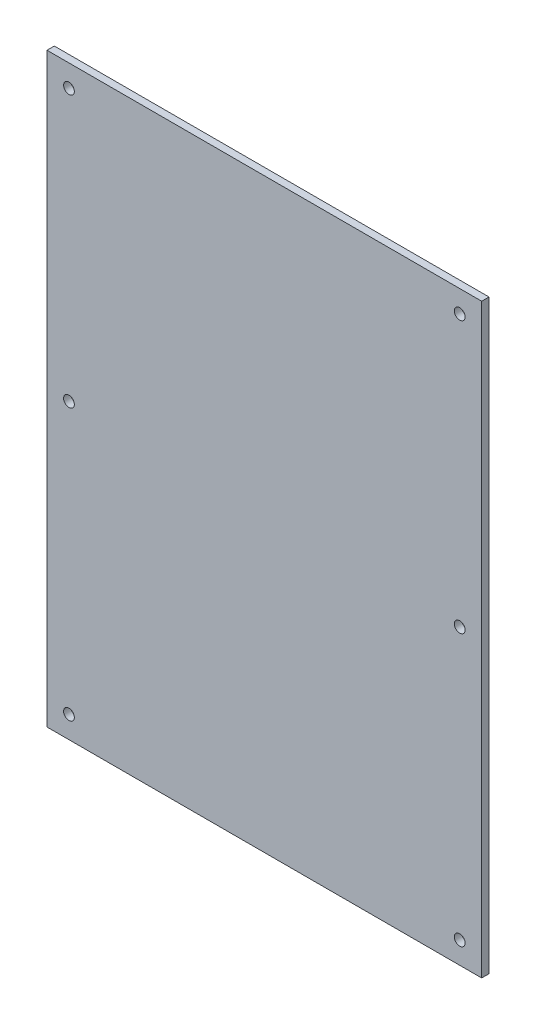
from build123d import *

# Parameters (mm, degrees)
SKETCH_1_W          = 178
SKETCH_1_H          = 240
EXTRUDE_1_DEPTH     = 3
SKETCH_2_R          = 2.2
CUT_EXTRUDE_1_DEPTH = 10


with BuildPart() as part:
    # 草图1 → 凸台-拉伸1 (new body)
    with BuildSketch(Plane.XY):
        Rectangle(SKETCH_1_W, SKETCH_1_H)
    extrude(amount=EXTRUDE_1_DEPTH)

    # 草图2 → 切除-拉伸1 (cut)
    with BuildSketch(Plane.XY.offset(3)):
        with Locations((-80, 111)):
            Circle(SKETCH_2_R)
        with Locations((80, 111)):
            Circle(SKETCH_2_R)
        with Locations((80, -111)):
            Circle(SKETCH_2_R)
        with Locations((-80, -111)):
            Circle(SKETCH_2_R)
        with Locations((-80, 0)):
            Circle(SKETCH_2_R)
        with Locations((80, 0)):
            Circle(SKETCH_2_R)
    extrude(amount=-CUT_EXTRUDE_1_DEPTH, mode=Mode.SUBTRACT)


solid = part.part
